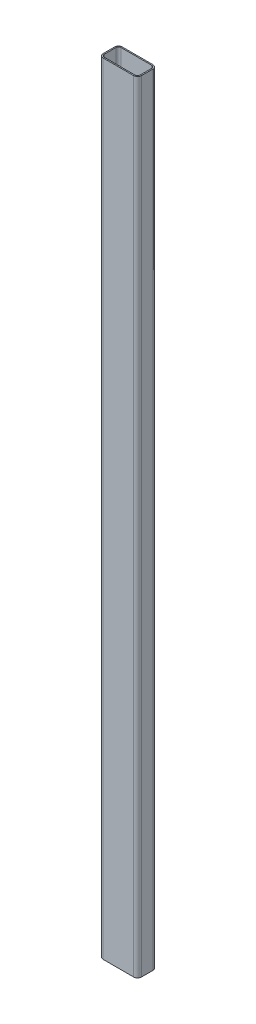
SolidWorks part; units mm, degrees
ref_plane "Front Plane" through (0, 0, 0) normal (0, 0, 1) x (1, 0, 0)
ref_plane "Top Plane" through (0, 0, 0) normal (0, 1, 0) x (1, 0, 0)
ref_plane "Right Plane" through (0, 0, 0) normal (1, 0, 0) x (0, 0, -1)
other "Configuration Table"
sketch "Sketch1" plane through (0, 0, 0) normal (0, 1, 0) x (1, 0, 0)
  line L1 (-40, 25) -> (40, 25)
  line L2 (-50, 15) -> (-50, -15)
  line L3 (-40, -25) -> (40, -25)
  line L4 (50, 15) -> (50, -15)
  line L5 (-50, 25) -> (50, -25) construction
  line L6 (-50, -25) -> (50, 25) construction
  arc A0 (40, 25) -> (50, 15) centre (40, 15) cw
  arc A1 (40, -25) -> (50, -15) centre (40, -15) ccw
  arc A2 (-50, -15) -> (-40, -25) centre (-40, -15) ccw
  arc A3 (-40, 25) -> (-50, 15) centre (-40, 15) ccw
  point P0 (0, 0)
  dimension "D3" = 10
  dimension "D1" = 100
  dimension "D2" = 50
extrude "Extrude-Thin1" add sketch "Sketch1" along normal mid plane 2040 thin
